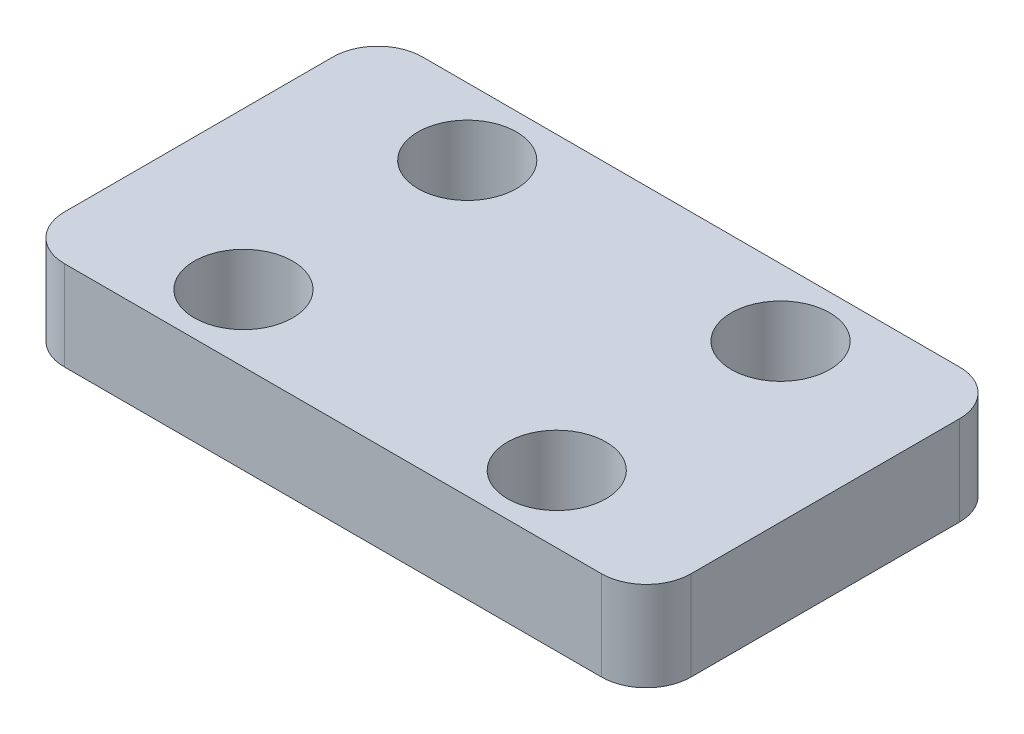
from build123d import *

# Parameters (mm, degrees)
SKETCH_1_W          = 70
SKETCH_1_H          = 40
EXTRUDE_1_DEPTH     = 5
HOLE_WIZARD_M10_1_D = 11
FILLET_1_R          = 5


with BuildPart() as part:
    # 草图1 → 凸台-拉伸1 (new, symmetric)
    with BuildSketch(Plane(origin=(0, 0, 0), x_dir=(1, 0, 0), z_dir=(0, 1, 0))):
        Rectangle(SKETCH_1_W, SKETCH_1_H)
    extrude(amount=EXTRUDE_1_DEPTH, both=True)

    # M10 间隙孔1 (through all)
    with Locations(Plane(origin=(0, 5, 0), x_dir=(1, 0, 0), z_dir=(0, 1, 0))):
        with Locations((-17.5, 12.5), (17.5, 12.5), (17.5, -12.5), (-17.5, -12.5)):
            Hole(HOLE_WIZARD_M10_1_D / 2)

    # 圆角1
    fillet_1_edges = [part.edges().sort_by_distance(p)[0] for p in [
        (35, 0, 20),
        (-35, 0, 20),
        (-35, 0, -20),
        (35, 0, -20),
    ]]
    fillet(fillet_1_edges, radius=FILLET_1_R)


solid = part.part
